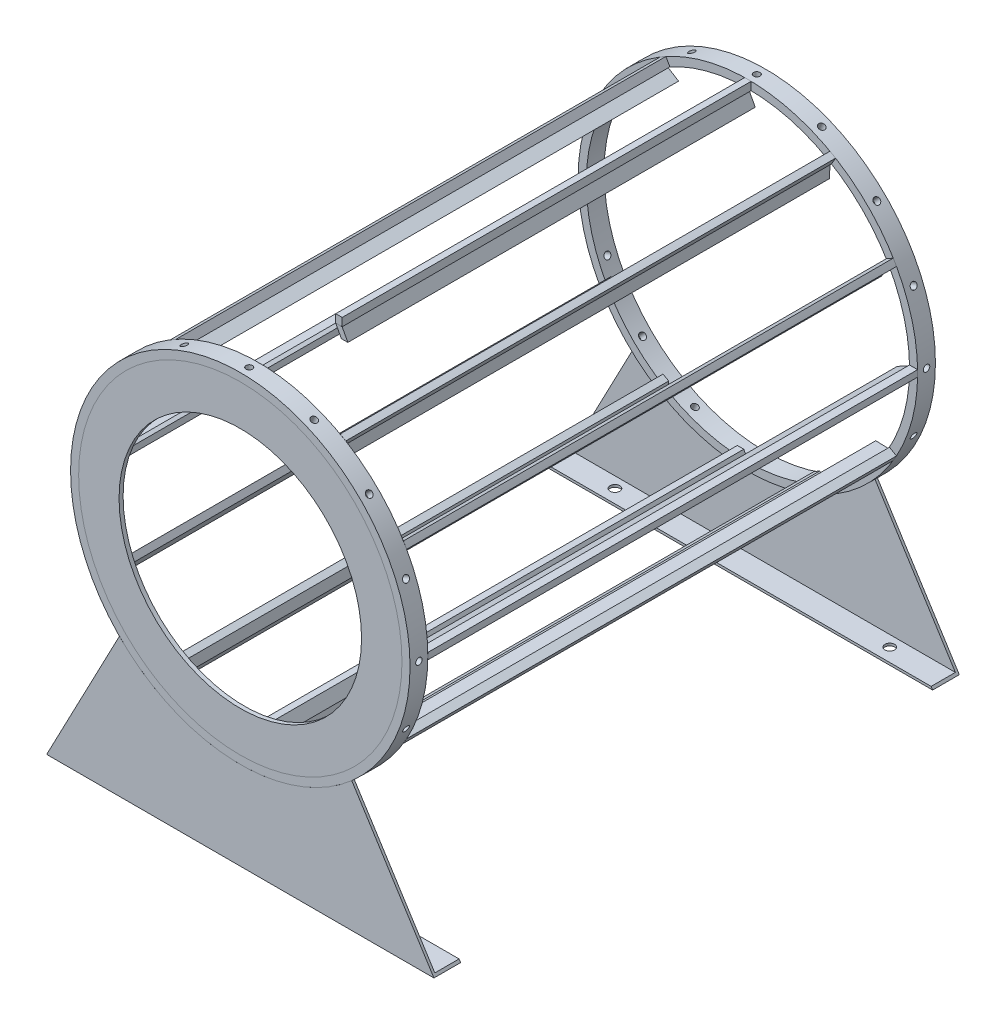
SolidWorks part; units mm, degrees
ref_plane "前视基准面" through (0, 0, 0) normal (0, 0, 1) x (1, 0, 0)
ref_plane "上视基准面" through (0, 0, 0) normal (0, 1, 0) x (1, 0, 0)
ref_plane "右视基准面" through (0, 0, 0) normal (1, 0, 0) x (0, 0, -1)
sketch "草图1" plane through (0, 0, 0) normal (0, 0, 1) x (1, 0, 0)
  circle A0 centre (0, 0) radius 210
  circle A1 centre (0, 0) radius 200
  dimension "D1" = 420
  dimension "D2" = 10
extrude "凸台-拉伸1" add sketch "草图1" against normal blind 22
ref_plane "基准面1" through (0, 0, -325) normal (0, 0, 1) x (1, 0, 0)
sketch "草图2" plane through (0, 0, 0) normal (0, 1, 0) x (1, 0, 0)
  line L0 (0, 0) -> (0, 11) construction
  circle A0 centre (0, 11) radius 4
  dimension "D2" = 8
  dimension "D1" = 11
extrude "切除-拉伸1" cut sketch "草图2" along normal through all
pattern_circular "阵列(圆周)1" count 16 every 22.5 about axis through (0, 0, 0) along (0, 0, 1) of "切除-拉伸1"
mirror "镜向7" about plane through (0, 0, -325) normal (0, 0, 1) of bodies 109
sketch "草图3" plane through (0, 0, -325) normal (0, 0, 1) x (1, 0, 0)
  line L0 (0, 0) -> (0, 254.8039) construction
  line L1 (4, 199.96) -> (4, 209.9619)
  line L2 (-4, 199.96) -> (-4, 209.9619)
  line L4 (4, 0) -> (4, 254.8039) construction
  line L5 (-4, 0) -> (-4, 254.8039) construction
  circle A0 centre (0, 0) radius 200 construction
  circle A1 centre (0, 0) radius 210
  arc A2 (4, 209.9619) -> (-4, 209.9619) centre (0, 0) ccw
  arc A3 (4, 199.96) -> (-4, 199.96) centre (0, 0) ccw
  dimension "D1" = 4
  dimension "D2" = 4
  dimension "D3" = 0
extrude "凸台-拉伸2" add sketch "草图3" along normal mid plane 606 separate body
sketch "草图4" plane through (0, 0, -325) normal (0, 0, 1) x (1, 0, 0)
  line L0 (4, 199.96) -> (11.0768, 186.7343)
  line L1 (-4, 199.96) -> (3.0768, 186.7343)
  line L2 (3.0768, 186.7343) -> (11.0768, 186.7343)
  line L3 (-4, 199.96) -> (4, 199.96)
  dimension "D1" = 15
extrude "凸台-拉伸3" add sketch "草图4" along normal mid plane 602 separate body
pattern_circular "阵列(圆周)5" count 12 every 30 about axis through (0, 0, 0) along (0, 0, 1) of bodies 135 111
sketch "草图5" plane through (0, 0, 0) normal (0, 1, 0) x (1, 0, 0)
  line L0 (210, 22) -> (-210, 22) construction
  line L1 (-18.4052, 22) -> (24.6379, 22)
  line L2 (-18.4052, 22) -> (-18.4052, 122)
  line L3 (-18.4052, 122) -> (24.6379, 122)
  line L4 (24.6379, 22) -> (24.6379, 122)
  dimension "D1" = 100
extrude "切除-拉伸2" cut sketch "草图5" along normal blind 602
sketch "草图6" plane through (0, 0, -650) normal (0, 0, -1) x (-1, 0, 0)
  line L0 (-137.9136, -158.3662) -> (-239.5557, -319)
  line L1 (0, 0) -> (0, -423.464) construction
  line L2 (149.5625, -147.4146) -> (239.5557, -319)
  line L3 (-239.5557, -319) -> (239.5557, -319)
  circle A2 centre (0, 0) radius 210 construction
  arc A3 (-137.9136, -158.3662) -> (149.5625, -147.4146) centre (0, 0) ccw
  dimension "D1" = 319
  dimension "D2" = 60
extrude "凸台-拉伸4" add sketch "草图6" against normal blind 3 separate body
sketch "草图7" plane through (0, 0, -647) normal (0, 0, 1) x (1, 0, 0)
  line L0 (239.5557, -319) -> (-239.5557, -319) construction
  line L1 (239.5557, -319) -> (-239.5557, -319)
  line L2 (239.5557, -316) -> (-239.5557, -316)
  line L3 (-239.5557, -316) -> (-239.5557, -319)
  line L4 (239.5557, -315.6559) -> (239.5557, -319)
  line M1 (-239.5557, -319) -> (239.5557, -319)
  line M2 (239.5557, -319) -> (137.9136, -158.3662)
  line M4 (-149.5625, -147.4146) -> (-239.5557, -319)
  dimension "D1" = 3
extrude "凸台-拉伸5" add sketch "草图7" along normal blind 30 contours L2 M2 M4 M1
sketch "草图8" plane through (0, -319, 0) normal (0, -1, 0) x (1, 0, 0)
  line L0 (-239.5557, -633.5) -> (239.5557, -633.5) construction
  line L1 (-239.5557, -617) -> (-239.5557, -650) construction
  line L2 (239.5557, -617) -> (239.5557, -650) construction
  line L3 (0, -650) -> (0, -617) construction
  line L4 (239.5557, -650) -> (-239.5557, -650) construction
  line L5 (-239.5557, -617) -> (239.5557, -617) construction
  circle A0 centre (-170, -633.5) radius 6
  circle A1 centre (170, -633.5) radius 6
  dimension "D1" = 12
  dimension "D2" = 170
extrude "切除-拉伸3" cut sketch "草图8" against normal blind 10
mirror "镜向10" about plane through (0, 0, -325) normal (0, 0, 1)
sketch "草图9" plane through (0, 0, 0) normal (0, 0, 1) x (1, 0, 0)
  circle A0 centre (0, 0) radius 150
  circle A1 centre (0, 0) radius 200 construction
  circle A2 centre (0, 0) radius 200
  dimension "D1" = 300
extrude "凸台-拉伸6" add sketch "草图9" against normal blind 5 separate body
